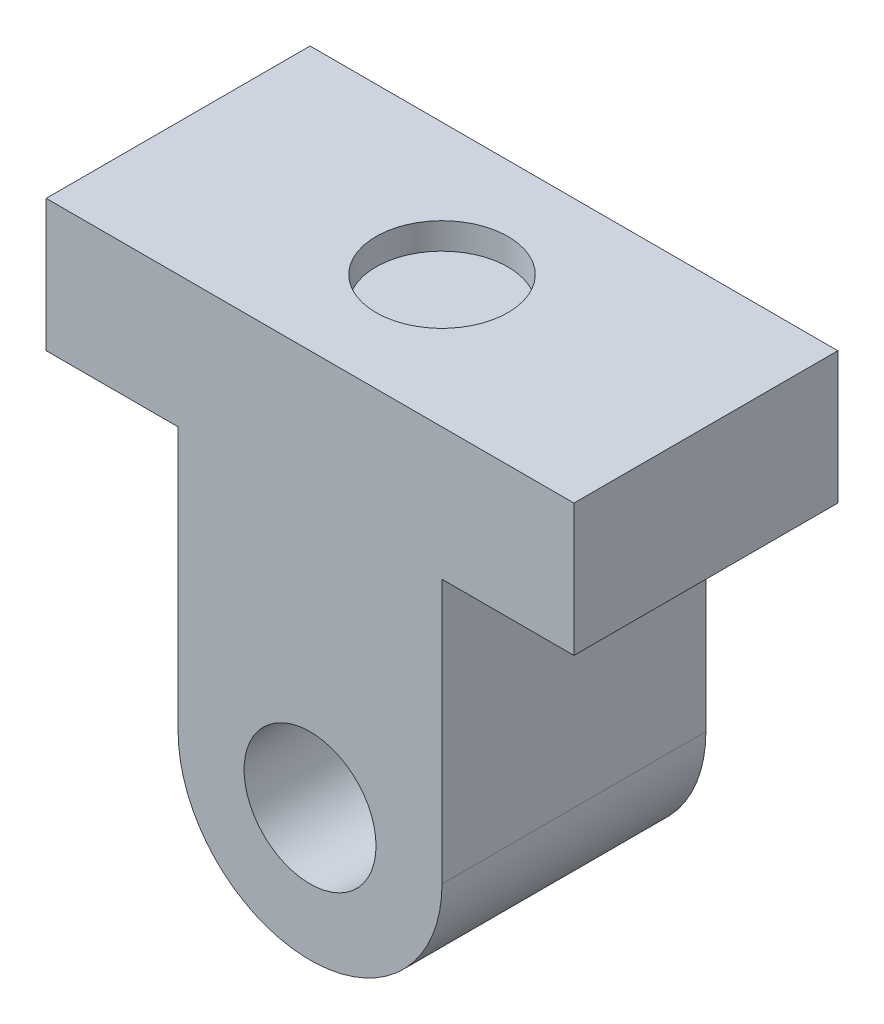
SolidWorks part; units mm, degrees
ref_plane "Front Plane" through (0, 0, 0) normal (0, 0, 1) x (1, 0, 0)
ref_plane "Top Plane" through (0, 0, 0) normal (0, 1, 0) x (1, 0, 0)
ref_plane "Right Plane" through (0, 0, 0) normal (1, 0, 0) x (0, 0, -1)
other "Configuration Table"
sketch "Sketch1" plane through (0, 0, 0) normal (0, 0, 1) x (1, 0, 0)
  line L0 (-5, 0) -> (-5, 10)
  line L1 (-5, 10) -> (-10, 10)
  line L2 (-10, 10) -> (-10, 15)
  line L3 (-10, 15) -> (10, 15)
  line L4 (0, 0) -> (0, 15) construction
  line L5 (5, 0) -> (5, 10)
  line L6 (5, 10) -> (10, 10)
  line L7 (10, 10) -> (10, 15)
  circle A0 centre (0, 0) radius 2.5
  arc A1 (-5, 0) -> (5, 0) centre (0, 0) ccw
  dimension "D1" = 5
  dimension "D2" = 10
  dimension "D3" = 10
  dimension "D4" = 5
  dimension "D5" = 10
extrude "Boss-Extrude1" add sketch "Sketch1" along normal blind 10
sketch "Sketch2" plane through (0, 15, 0) normal (0, 1, 0) x (1, 0, 0)
  line L0 (10, -10) -> (-10, -10) construction
  circle A2 centre (0, -5) radius 2.5
  dimension "D1" = 5
  dimension "D2" = 5
extrude "Cut-Extrude1" cut sketch "Sketch2" against normal blind 1
